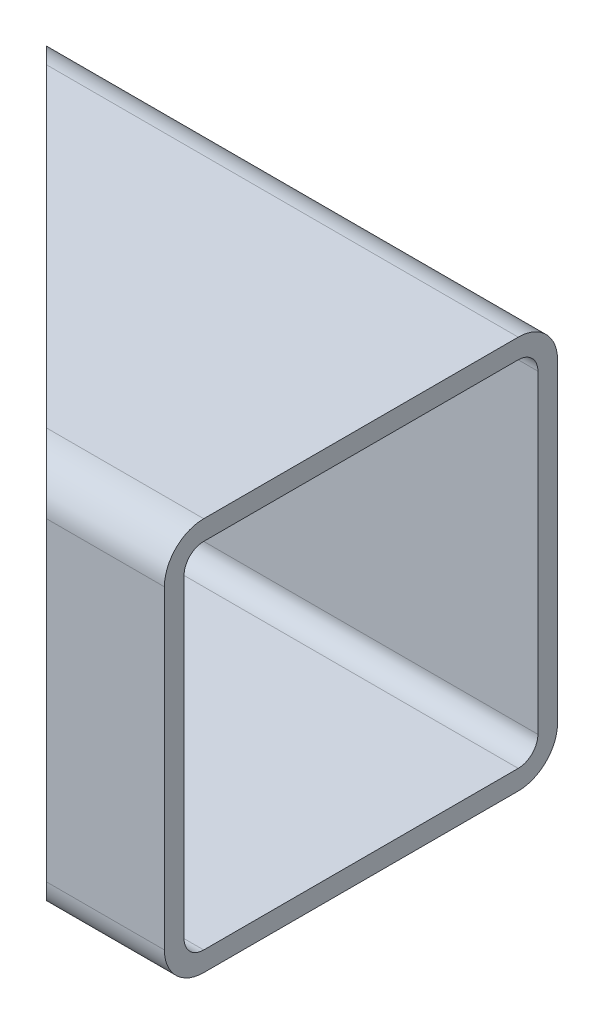
SolidWorks part; units mm, degrees
material "普通碳钢"
ref_plane "前视基准面" through (0, 0, 0) normal (0, 0, 1) x (1, 0, 0)
ref_plane "上视基准面" through (0, 0, 0) normal (0, 1, 0) x (1, 0, 0)
ref_plane "右视基准面" through (0, 0, 0) normal (1, 0, 0) x (0, 0, -1)
sketch3d "3D草图1"
  line L0 (0, 0, 0) -> (200, 0, 0)
  dimension "D1" = 200
other "方形管 100 X 100 X 5   (1)"
ref_plane "基准面1" through (0, 0, 0) normal (1, 0, 0) x (0, 0, -1)
sketch "Sketch1" plane through (0, 0, 0) normal (1, 0, 0) x (0, 0, -1)
  line L0 (-40, -45) -> (40, -45)
  line L1 (-45, -40) -> (-45, 40)
  line L2 (40, 45) -> (-40, 45)
  line L3 (45, 40) -> (45, -40)
  line L4 (-40, -50) -> (40, -50)
  line L5 (-50, -40) -> (-50, 40)
  line L6 (40, 50) -> (-40, 50)
  line L7 (50, 40) -> (50, -40)
  arc A0 (50, 40) -> (40, 50) centre (40, 40) ccw
  arc A1 (40, -50) -> (50, -40) centre (40, -40) ccw
  arc A2 (-50, -40) -> (-40, -50) centre (-40, -40) ccw
  arc A3 (-40, 50) -> (-50, 40) centre (-40, 40) ccw
  arc A4 (-40, 45) -> (-45, 40) centre (-40, 40) ccw
  arc A5 (45, 40) -> (40, 45) centre (40, 40) ccw
  arc A6 (40, -45) -> (45, -40) centre (40, -40) ccw
  arc A7 (-45, -40) -> (-40, -45) centre (-40, -40) ccw
  point P0 (-50, 0)
  point P1 (50, 0)
  point P2 (0, 50)
  point P3 (0, -50)
  point P4 (0, 0)
  point P5 (-50, -50)
  point P6 (50, -50)
  point P7 (50, 50)
  point P8 (-50, 50)
  point P33 (0, 0)
  dimension "D1" = 10
  dimension "Thickness" = 5
  dimension "V_leg" = 100
sketch "草图2" plane through (0, 50, 0) normal (0, -1, 0) x (1, 0, 0)
  line L3 (170, 50) -> (70, -50)
  line L4 (200, 50) -> (0, 50) construction
  line L5 (200, -50) -> (0, -50) construction
  line L7 (70, -50) -> (0, -50)
  line L8 (0, -50) -> (0, 50)
  line L9 (200, 40) -> (200, 50) construction
  line L10 (0, 50) -> (170, 50)
  dimension "D1" = 30
  dimension "D2" = 45
extrude "切除-拉伸1" cut sketch "草图2" along normal up to surface (100 mm away) up to face at (100, -50, 0)
